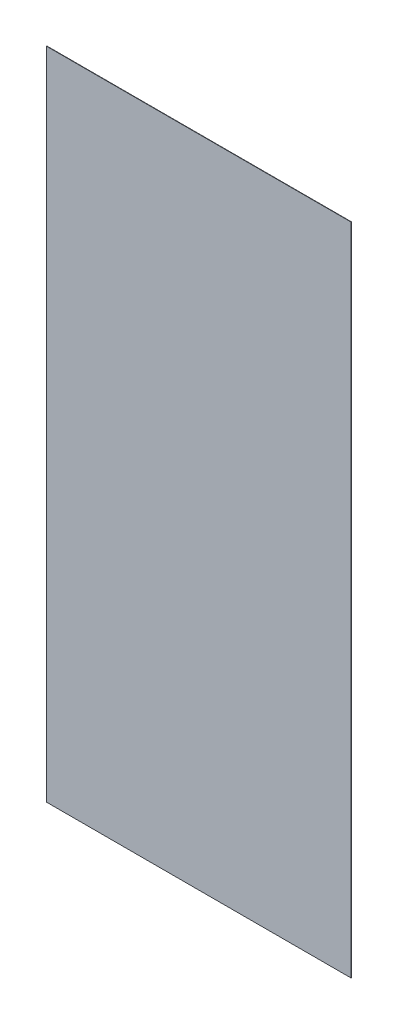
from build123d import *

# Parameters (mm, degrees)
SKETCH1_W           = 800
SKETCH1_H           = 1720
BOSS_EXTRUDE1_DEPTH = 1


with BuildPart() as part:
    # Sketch1 → Boss-Extrude1 (new body)
    with BuildSketch(Plane.XY):
        Rectangle(SKETCH1_W, SKETCH1_H)
    extrude(amount=BOSS_EXTRUDE1_DEPTH)


solid = part.part
